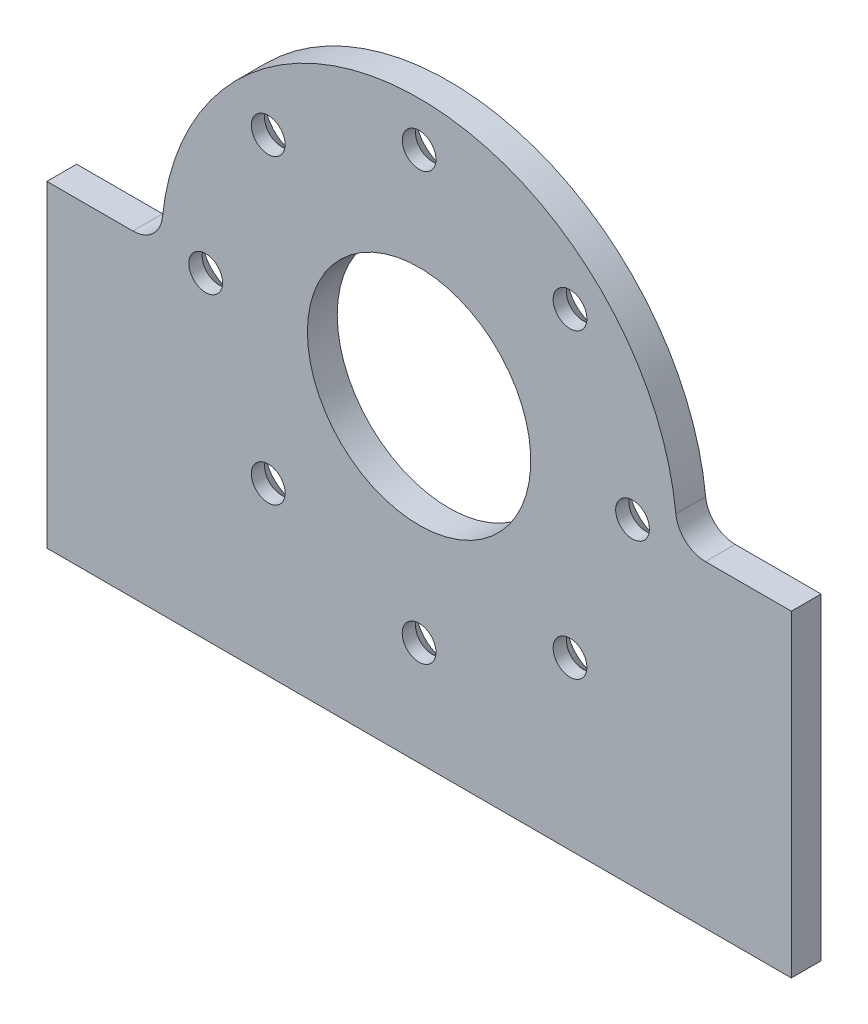
SolidWorks part; units mm, degrees
material "SUS304"
ref_plane "前视基准面" through (0, 0, 0) normal (0, 0, 1) x (1, 0, 0)
ref_plane "上视基准面" through (0, 0, 0) normal (0, 1, 0) x (1, 0, 0)
ref_plane "右视基准面" through (0, 0, 0) normal (1, 0, 0) x (0, 0, -1)
sketch "草图1" plane through (0, 0, 0) normal (0, 0, 1) x (1, 0, 0)
  line L1 (-37.5, -16) -> (37.5, -16)
  line L2 (-37.5, -16) -> (-37.5, 16)
  line L3 (-37.5, 16) -> (37.5, 16)
  line L4 (37.5, -16) -> (37.5, 16)
  line L5 (-37.5, -16) -> (37.5, 16) construction
  line L6 (-37.5, 16) -> (37.5, -16) construction
  point P0 (0, 0)
  dimension "D1" = 32
  dimension "D2" = 75
extrude "凸台-拉伸1" add sketch "草图1" along normal blind 3
sketch "草图2" plane through (0, 0, 3) normal (0, 0, 1) x (1, 0, 0)
  line L1 (-37.5, -16) -> (37.5, -16) construction
  circle A0 centre (0, 16) radius 26
  dimension "D1" = 52
  dimension "D2" = 32
extrude "凸台-拉伸3" add sketch "草图2" against normal through all
fillet "圆角1" radius 3 2 edges at (26, 16, 1.5) (-26, 16, 1.5)
sketch "草图3" plane through (0, 0, 0) normal (0, 0, -1) x (-1, 0, 0)
  circle A0 centre (0, 16) radius 11.25
  dimension "D1" = 22.5
extrude "切除-拉伸1" cut sketch "草图3" against normal through all
hole_wizard "M3 六角凹锥坑螺钉的锥形沉头孔1" positions "草图4" profile "草图5" countersink size "M3" standard "ISO" end condition through all
sketch "草图4" plane through (0, 0, 0) normal (0, 0, -1) x (-1, 0, 0)
  line L0 (0, 37.5) -> (0, 16) construction
  line L2 (0, 16) -> (0, 37.5) construction
  point P0 (0, 37.5)
  point P36 (15.2028, 31.2028)
  point P37 (21.5, 16)
  point P38 (15.2028, 0.7972)
  point P39 (0, -5.5)
  point P40 (-15.2028, 0.7972)
  point P41 (-21.5, 16)
  point P42 (-15.2028, 31.2028)
  dimension "D1" = 21.5
  dimension "D2" = 8
sketch "草图5" plane through (0, 37.5, 0) normal (1, 0, 0) x (0, 1, 0)
  line L0 (0, 0) -> (0, 3)
  line L1 (0, 3) -> (1.7, 3)
  line L2 (1.7, 3) -> (1.7, 1.66)
  line L3 (1.7, 1.66) -> (3.36, 0)
  line L5 (3.36, 0) -> (0, 0)
  line L6 (-1.7, 1.66) -> (-3.36, 0) construction
  line L11 (0, -6.35) -> (0, 107.95) construction
  dimension "通孔孔直径" = 3.4
  dimension "通孔孔深度" = 3
  dimension "近端锥形沉头孔直径" = 6.72
  dimension "近端锥形沉头孔角度" = 90
